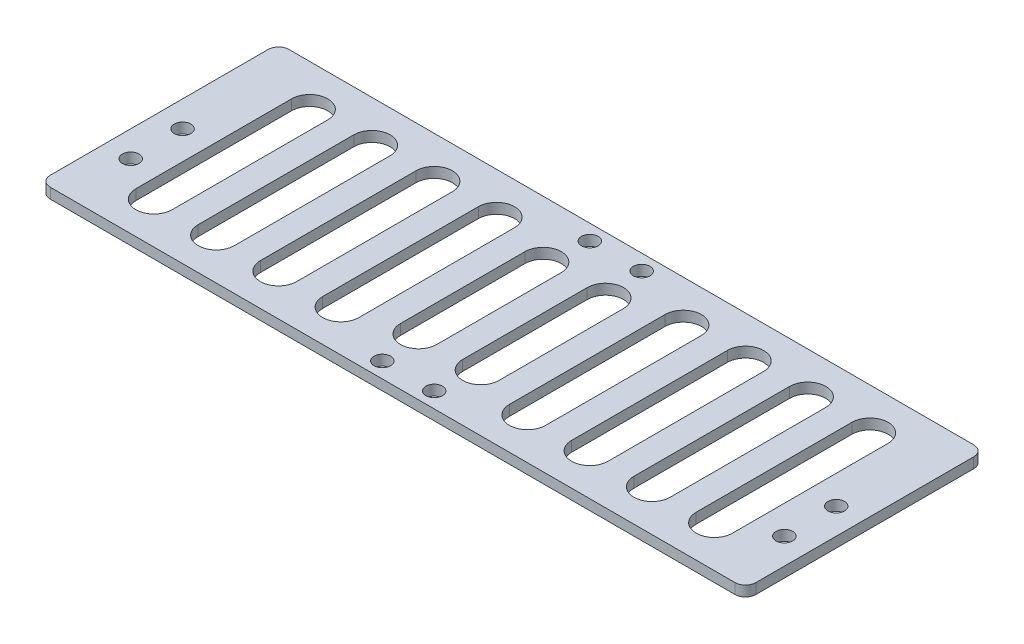
from build123d import *

# Parameters (mm, degrees)
SKETCH1_W           = 136
SKETCH1_H           = 46
SKETCH1_R           = 1.6
BOSS_EXTRUDE1_DEPTH = 2
CUT_EXTRUDE1_DEPTH  = 72.812255222
R2_FILLET_1_R       = 2


with BuildPart() as part:
    # Sketch1 → Boss-Extrude1 (new body)
    with BuildSketch(Plane(origin=(0, 0, 0), x_dir=(1, 0, 0), z_dir=(0, 1, 0))):
        Rectangle(SKETCH1_W, SKETCH1_H)
        with Locations(Location((-63, -0.5, 0), (0, 0, 270))):
            Circle(SKETCH1_R, mode=Mode.SUBTRACT)
        with Locations(Location((-63, -10.5, 0), (0, 0, 270))):
            Circle(SKETCH1_R, mode=Mode.SUBTRACT)
        with Locations(Location((-5, -20, 0), (0, 0, 270))):
            Circle(SKETCH1_R, mode=Mode.SUBTRACT)
        with Locations(Location((5, -20, 0), (0, 0, 270))):
            Circle(SKETCH1_R, mode=Mode.SUBTRACT)
        with Locations(Location((63, -10.5, 0), (0, 0, 90))):
            Circle(SKETCH1_R, mode=Mode.SUBTRACT)
        with Locations(Location((63, -0.5, 0), (0, 0, 90))):
            Circle(SKETCH1_R, mode=Mode.SUBTRACT)
        with Locations(Location((5, 20, 0), (0, 0, 90))):
            Circle(SKETCH1_R, mode=Mode.SUBTRACT)
        with Locations(Location((-5, 20, 0), (0, 0, 90))):
            Circle(SKETCH1_R, mode=Mode.SUBTRACT)
    extrude(amount=BOSS_EXTRUDE1_DEPTH)

    # Sketch2 → Cut-Extrude1 (cut, through all)
    with BuildSketch(Plane(origin=(0, 2, 0), x_dir=(1, 0, 0), z_dir=(0, 1, 0))):
        with BuildLine():
            Line((-50.5, 15), (-50.5, -15))
            ThreePointArc((-50.5, -15), (-54, -18.5), (-57.5, -15))
            Line((-57.5, -15), (-57.5, 15))
            ThreePointArc((-57.5, 15), (-54, 18.5), (-50.5, 15))
        make_face()
        with BuildLine():
            Line((-38.5, 15), (-38.5, -15))
            ThreePointArc((-38.5, -15), (-42, -18.5), (-45.5, -15))
            Line((-45.5, -15), (-45.5, 15))
            ThreePointArc((-45.5, 15), (-42, 18.5), (-38.5, 15))
        make_face()
        with BuildLine():
            Line((-26.5, 15), (-26.5, -15))
            ThreePointArc((-26.5, -15), (-30, -18.5), (-33.5, -15))
            Line((-33.5, -15), (-33.5, 15))
            ThreePointArc((-33.5, 15), (-30, 18.5), (-26.5, 15))
        make_face()
        with BuildLine():
            Line((-14.5, 15), (-14.5, -15))
            ThreePointArc((-14.5, -15), (-18, -18.5), (-21.5, -15))
            Line((-21.5, -15), (-21.5, 15))
            ThreePointArc((-21.5, 15), (-18, 18.5), (-14.5, 15))
        make_face()
        with BuildLine():
            Line((-2.5, 12), (-2.5, -12))
            ThreePointArc((-2.5, -12), (-6, -15.5), (-9.5, -12))
            Line((-9.5, -12), (-9.5, 12))
            ThreePointArc((-9.5, 12), (-6, 15.5), (-2.5, 12))
        make_face()
        with BuildLine():
            Line((9.5, 12), (9.5, -12))
            ThreePointArc((9.5, -12), (6, -15.5), (2.5, -12))
            Line((2.5, -12), (2.5, 12))
            ThreePointArc((2.5, 12), (6, 15.5), (9.5, 12))
        make_face()
        with BuildLine():
            Line((21.5, 15), (21.5, -15))
            ThreePointArc((21.5, -15), (18, -18.5), (14.5, -15))
            Line((14.5, -15), (14.5, 15))
            ThreePointArc((14.5, 15), (18, 18.5), (21.5, 15))
        make_face()
        with BuildLine():
            Line((33.5, 15), (33.5, -15))
            ThreePointArc((33.5, -15), (30, -18.5), (26.5, -15))
            Line((26.5, -15), (26.5, 15))
            ThreePointArc((26.5, 15), (30, 18.5), (33.5, 15))
        make_face()
        with BuildLine():
            Line((45.5, 15), (45.5, -15))
            ThreePointArc((45.5, -15), (42, -18.5), (38.5, -15))
            Line((38.5, -15), (38.5, 15))
            ThreePointArc((38.5, 15), (42, 18.5), (45.5, 15))
        make_face()
        with BuildLine():
            Line((57.5, 15), (57.5, -15))
            ThreePointArc((57.5, -15), (54, -18.5), (50.5, -15))
            Line((50.5, -15), (50.5, 15))
            ThreePointArc((50.5, 15), (54, 18.5), (57.5, 15))
        make_face()
    extrude(amount=-CUT_EXTRUDE1_DEPTH, mode=Mode.SUBTRACT)

    # R2 Fillet 1
    r2_fillet_1_edges = [part.edges().sort_by_distance(p)[0] for p in [
        (-68, 1, -23),
        (68, 1, -23),
        (68, 1, 23),
        (-68, 1, 23),
    ]]
    fillet(r2_fillet_1_edges, radius=R2_FILLET_1_R)


solid = part.part
